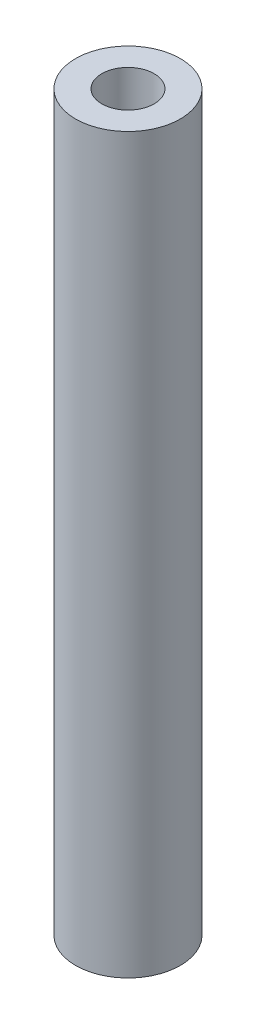
from build123d import *

# Parameters (mm, degrees)
SKETCH1_R           = 20
SKETCH1_R_2         = 10
BOSS_EXTRUDE1_DEPTH = 140


with BuildPart() as part:
    # Sketch1 → Boss-Extrude1 (new, symmetric)
    with BuildSketch(Plane(origin=(0, 0, 0), x_dir=(1, 0, 0), z_dir=(0, 1, 0))):
        with Locations(Location((0, 0, 0), (0, 0, 270))):
            Circle(SKETCH1_R)
        with Locations(Location((0, 0, 0), (0, 0, 270))):
            Circle(SKETCH1_R_2, mode=Mode.SUBTRACT)
    extrude(amount=BOSS_EXTRUDE1_DEPTH, both=True)


solid = part.part
